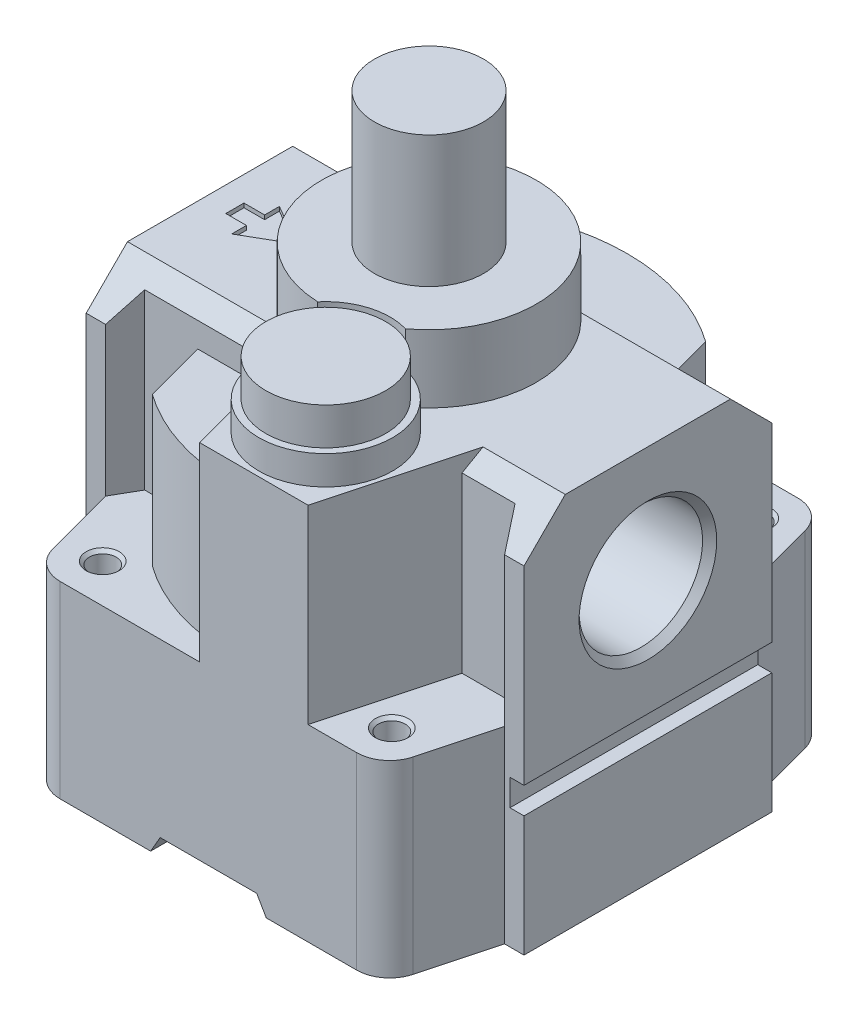
from build123d import *

# Parameters (mm, degrees)
EXTRUDE_1_DEPTH             = 22.8
EXTRUDE_2_DEPTH             = 45.8
CUT_EXTRUDE_1_DEPTH         = 26.5
CUT_EXTRUDE_1_DEPTH_BACK    = 26.5
EXTRUDE_3_DEPTH             = 40.8
CUT_EXTRUDE_2_DEPTH         = 26.7
CUT_EXTRUDE_2_DEPTH_BACK    = 26.7
SKETCH_5_W                  = 1.7
SKETCH_5_H                  = 3.2
CUT_EXTRUDE_3_DEPTH         = 26.7
CUT_EXTRUDE_3_DEPTH_BACK    = 26.7
SKETCH_6_W                  = 1.7
SKETCH_6_H                  = 3.2
HOLE_WIZARD_1_D             = 14.95
HOLE_WIZARD_1_DEPTH         = 11.7
HOLE_WIZARD_1_CSINK_D       = 16.662
HOLE_WIZARD_1_CSINK_ANGLE   = 90
HOLE_WIZARD_1_TIP           = 4.315693262
HOLE_WIZARD_2_D             = 14.95
HOLE_WIZARD_2_DEPTH         = 11.7
HOLE_WIZARD_2_CSINK_D       = 16.662
HOLE_WIZARD_2_CSINK_ANGLE   = 90
HOLE_WIZARD_2_TIP           = 4.315693262
PATTERN_LINEAR_1_COUNT      = 2
PATTERN_LINEAR_1_PITCH      = 44
PATTERN_LINEAR_1_COUNT_DIR2 = 2
PATTERN_LINEAR_1_PITCH_DIR2 = 35
EXTRUDE_4_DEPTH             = 23
SKETCH_16_R                 = 7.8
CUT_EXTRUDE_4_DEPTH         = 8.2
SKETCH_17_R                 = 8.1
EXTRUDE_5_DEPTH             = 3.5
SKETCH_18_R                 = 7.25
EXTRUDE_6_DEPTH             = 4.5
CUT_EXTRUDE_5_DEPTH         = 0.5
CUT_EXTRUDE_6_DEPTH         = 26.7
CUT_EXTRUDE_6_DEPTH_BACK    = 26.7
SKETCH_21_W                 = 23
SKETCH_21_H                 = 2


with BuildPart() as part:
    # 草图1 → 凸台-拉伸1 (new body)
    with BuildSketch(Plane(origin=(0, -31.8, 0), x_dir=(1, 0, 0), z_dir=(0, 1, 0))):
        with BuildLine():
            Line((-24.15, -15), (-21.809389802, -23.73527618))
            ThreePointArc((-21.809389802, -23.73527618), (-20.380732213, -25.873413361), (-17.945686497, -26.7))
            Line((-17.945686497, -26.7), (17.945686497, -26.7))
            ThreePointArc((17.945686497, -26.7), (20.380732213, -25.873413361), (21.809389802, -23.73527618))
            Line((21.809389802, -23.73527618), (24.15, -15))
            Line((24.15, -15), (24.15, 15))
            Line((24.15, 15), (21.809389802, 23.73527618))
            ThreePointArc((21.809389802, 23.73527618), (20.380732213, 25.873413361), (17.945686497, 26.7))
            Line((17.945686497, 26.7), (-17.945686497, 26.7))
            ThreePointArc((-17.945686497, 26.7), (-20.380732213, 25.873413361), (-21.809389802, 23.73527618))
            Line((-21.809389802, 23.73527618), (-24.15, 15))
            Line((-24.15, 15), (-24.15, -15))
        make_face()
    extrude(amount=EXTRUDE_1_DEPTH)

    # 草图2 → 凸台-拉伸2 (add)
    with BuildSketch(Plane(origin=(0, -31.8, 0), x_dir=(1, 0, 0), z_dir=(0, 1, 0))):
        Polygon((-26.5, -15), (-24.15, -15), (-22.417949192, -12), (22.417949192, -12), (24.15, -15), (26.5, -15), (26.5, 15), (24.15, 15), (22.417949192, 12), (-22.417949192, 12), (-24.15, 15), (-26.5, 15), align=None)
    extrude(amount=EXTRUDE_2_DEPTH)

    # 草图3 → 切除-拉伸1 (cut, two sides: drawn at the far end of the back side and taken through both)
    with BuildSketch(Plane(origin=(0, 0, 0), x_dir=(0, 0, -1), z_dir=(1, 0, 0)).offset(-CUT_EXTRUDE_1_DEPTH_BACK)):
        Polygon((-26.7, 45.8), (-26.7, 0), (-15, 0), (-15, 9), (-10, 14), (10, 14), (15, 9), (15, 0), (26.7, 0), (26.7, 45.8), align=None)
    extrude(amount=CUT_EXTRUDE_1_DEPTH + CUT_EXTRUDE_1_DEPTH_BACK, mode=Mode.SUBTRACT)

    # 草图4 → 凸台-拉伸3 (add)
    with BuildSketch(Plane(origin=(0, -31.8, 0), x_dir=(1, 0, 0), z_dir=(0, 1, 0))):
        with BuildLine():
            Line((-16, -12), (-13.99021743, -19.500610664))
            ThreePointArc((-13.99021743, -19.500610664), (0, -24), (13.99021743, -19.500610664))
            Line((13.99021743, -19.500610664), (16, -12))
            Line((16, -12), (16, 12))
            Line((16, 12), (13.99021743, 19.500610664))
            ThreePointArc((13.99021743, 19.500610664), (0, 24), (-13.99021743, 19.500610664))
            Line((-13.99021743, 19.500610664), (-16, 12))
            Line((-16, 12), (-16, -12))
        make_face()
    extrude(amount=EXTRUDE_3_DEPTH)

    # 草图5 → 切除-拉伸2 (cut, two sides: drawn at the far end of the back side and taken through both)
    with BuildSketch(Plane.XY.offset(-CUT_EXTRUDE_2_DEPTH_BACK)):
        with Locations((25.65, -15.6)):
            Rectangle(SKETCH_5_W, SKETCH_5_H)
    extrude(amount=CUT_EXTRUDE_2_DEPTH + CUT_EXTRUDE_2_DEPTH_BACK, mode=Mode.SUBTRACT)

    # 草图6 → 切除-拉伸3 (cut, two sides: drawn at the far end of the back side and taken through both)
    with BuildSketch(Plane.XY.offset(-CUT_EXTRUDE_3_DEPTH_BACK)):
        with Locations((-25.65, -15.6)):
            Rectangle(SKETCH_6_W, SKETCH_6_H)
    extrude(amount=CUT_EXTRUDE_3_DEPTH + CUT_EXTRUDE_3_DEPTH_BACK, mode=Mode.SUBTRACT)

    # 孔1
    with Locations(Plane(origin=(26.5, 0, 0), x_dir=(0, 0, -1), z_dir=(1, 0, 0))):
        with Locations((0, 0)):
            CounterSinkHole(HOLE_WIZARD_1_D / 2, HOLE_WIZARD_1_CSINK_D / 2, depth=HOLE_WIZARD_1_DEPTH, counter_sink_angle=HOLE_WIZARD_1_CSINK_ANGLE)
            with Locations((0, 0, -(HOLE_WIZARD_1_DEPTH + HOLE_WIZARD_1_TIP / 2))):  # 120° drill point
                Cone(0, HOLE_WIZARD_1_D / 2, HOLE_WIZARD_1_TIP, mode=Mode.SUBTRACT)

    # 孔2
    with Locations(Plane.ZY.offset(26.5)):
        with Locations((0, 0)):
            CounterSinkHole(HOLE_WIZARD_2_D / 2, HOLE_WIZARD_2_CSINK_D / 2, depth=HOLE_WIZARD_2_DEPTH, counter_sink_angle=HOLE_WIZARD_2_CSINK_ANGLE)
            with Locations((0, 0, -(HOLE_WIZARD_2_DEPTH + HOLE_WIZARD_2_TIP / 2))):  # 120° drill point
                Cone(0, HOLE_WIZARD_2_D / 2, HOLE_WIZARD_2_TIP, mode=Mode.SUBTRACT)

    # 草图11 → 孔3 (revolve, cut)
    with BuildSketch(Plane(origin=(17.5, -9, 22), x_dir=(0, 0, 1), z_dir=(1, 0, 0))):
        Polygon((0, 0), (0, 4.935884786), (1.621, 4), (1.621, 0.379), (2, 0), align=None)
    hole_wizard_3 = revolve(axis=Axis((17.5, 5.308894879, 22), (0, -1, 0)), mode=Mode.SUBTRACT)

    # 阵列(线性)1: Hole Wizard 3 2 × 2
    with Locations(*[(-j * PATTERN_LINEAR_1_PITCH_DIR2, 0, -i * PATTERN_LINEAR_1_PITCH) for i in range(PATTERN_LINEAR_1_COUNT) for j in range(PATTERN_LINEAR_1_COUNT_DIR2) if (i, j) != (0, 0)]):
        add(hole_wizard_3, mode=Mode.SUBTRACT)

    # 草图14 → 旋转1 (revolve)
    with BuildSketch(Plane.XY, mode=Mode.PRIVATE) as revolve_1_sk:
        Polygon((0, 38.1), (6.6, 38.1), (6.6, 22.2), (13, 22.2), (13, 9), (0, 9), align=None)
    revolve(revolve_1_sk.sketch.rotate(Axis((0, 9, 0), (0, 1, 0)), 180), axis=Axis((0, 9, 0), (0, 1, 0)))

    # 草图15 → 凸台-拉伸4 (add)
    with BuildSketch(Plane(origin=(0, 14, 0), x_dir=(1, 0, 0), z_dir=(0, 1, 0))):
        Polygon((-6.339745962, -7), (-1.061146871, -26.7), (12.061146871, -26.7), (17.339745962, -7), align=None)
    extrude(amount=-EXTRUDE_4_DEPTH)

    # 草图16 → 切除-拉伸4 (cut)
    with BuildSketch(Plane(origin=(0, 14, 0), x_dir=(1, 0, 0), z_dir=(0, 1, 0))):
        with Locations((5.5, -18)):
            Circle(SKETCH_16_R)
    extrude(amount=CUT_EXTRUDE_4_DEPTH, mode=Mode.SUBTRACT)

    # 草图17 → 凸台-拉伸5 (add)
    with BuildSketch(Plane(origin=(0, 14, 0), x_dir=(1, 0, 0), z_dir=(0, 1, 0))):
        with Locations((5.5, -18)):
            Circle(SKETCH_17_R)
    extrude(amount=EXTRUDE_5_DEPTH)

    # 草图18 → 凸台-拉伸6 (add)
    with BuildSketch(Plane(origin=(0, 17.5, 0), x_dir=(1, 0, 0), z_dir=(0, 1, 0))):
        with Locations(Location((5.5, -18, 0), (0, 0, 270))):
            Circle(SKETCH_18_R)
    extrude(amount=EXTRUDE_6_DEPTH)

    # 草图19 → 切除-拉伸5 (cut)
    with BuildSketch(Plane(origin=(0, 14, 0), x_dir=(1, 0, 0), z_dir=(0, 1, 0))):
        Polygon((-23.5, -1.1), (-21, -1.1), (-21, -2.886751346), (-16, 0), (-21, 2.886751346), (-21, 1.1), (-23.5, 1.1), align=None)
    extrude(amount=-CUT_EXTRUDE_5_DEPTH, mode=Mode.SUBTRACT)

    # 草图20 → 切除-拉伸6 (cut, two sides: drawn at the far end of the back side and taken through both)
    with BuildSketch(Plane.XY.offset(-CUT_EXTRUDE_6_DEPTH_BACK)):
        Polygon((-7, -31.8), (7, -31.8), (5.845299462, -29.8), (-5.845299462, -29.8), align=None)
    extrude(amount=CUT_EXTRUDE_6_DEPTH + CUT_EXTRUDE_6_DEPTH_BACK, mode=Mode.SUBTRACT)

    # 草图21 → 旋转2 (revolve)
    with BuildSketch(Plane.XY):
        with Locations((11.5, -30.8)):
            Rectangle(SKETCH_21_W, SKETCH_21_H)
    revolve(axis=Axis((0, -31.8, 0), (0, 1, 0)))


solid = part.part
